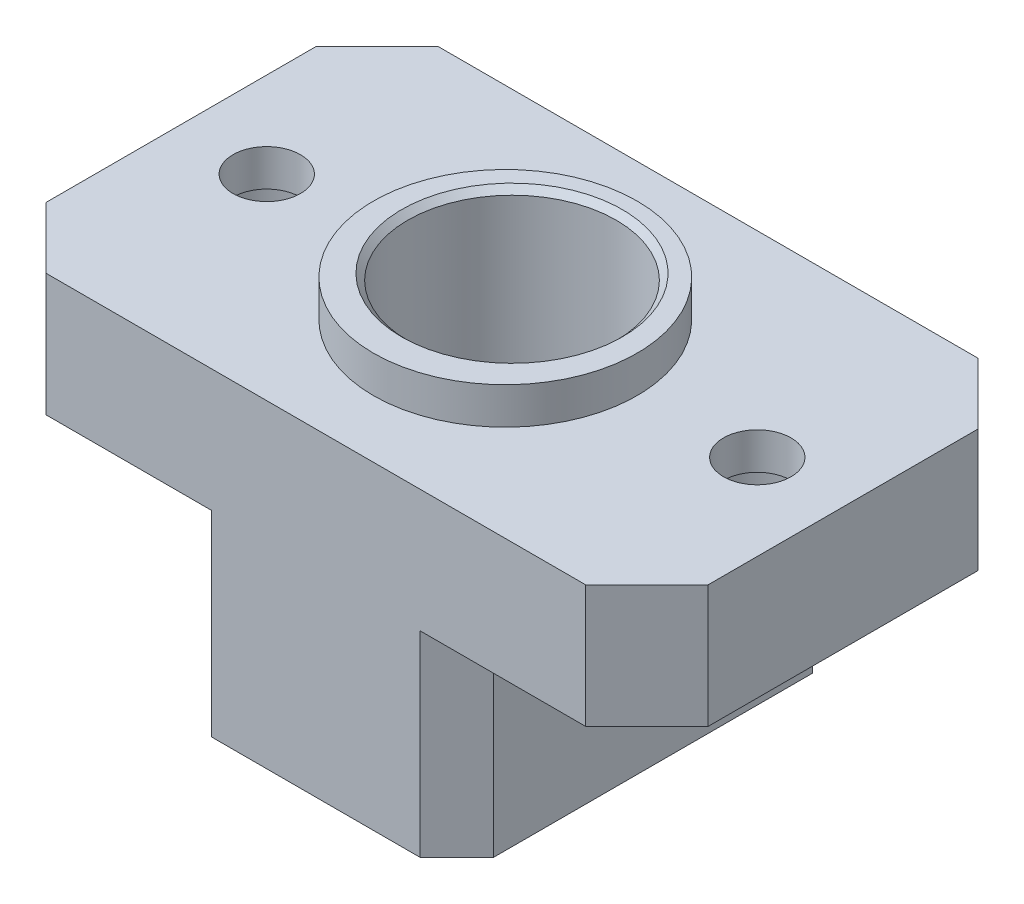
from build123d import *

# Parameters (mm, degrees)
BOSS_EXTRUDE1_DEPTH = 32
CHAMFER1_SIZE       = 5
SKETCH2_R           = 10.75
BOSS_EXTRUDE2_DEPTH = 3
HOLE2_D             = 5.5
HOLE2_DEPTH         = 100
HOLE2_CBORE_D       = 10
HOLE2_CBORE_DEPTH   = 7
CHAMFER3_SIZE       = 3
HOLE3_D             = 17
CHAMFER5_SIZE       = 0.5
CHAMFER6_SIZE       = 1


with BuildPart() as part:
    # Sketch1 → Boss-Extrude1 (new body)
    with BuildSketch(Plane.XY):
        Polygon((11.5, -16.008629624), (-11.5, -16.008629624), (-11.5, -0.008629624), (-27, -0.008629624), (-27, 9.991370376), (27, 9.991370376), (27, -0.008629624), (11.5, -0.008629624), align=None)
    extrude(amount=BOSS_EXTRUDE1_DEPTH)

    # Chamfer1
    chamfer1_edges = [part.edges().sort_by_distance(p)[0] for p in [
        (-27, 4.991370376, 0),
        (27, 4.991370376, 0),
        (-27, 4.991370376, 32),
        (27, 4.991370376, 32),
    ]]
    chamfer(chamfer1_edges, length=CHAMFER1_SIZE)

    # Sketch2 → Boss-Extrude2 (add)
    with BuildSketch(Plane(origin=(0, 9.991370376, 0), x_dir=(1, 0, 0), z_dir=(0, 1, 0))):
        with Locations(Location((0, -16.547126345, 0), (0, 0, 270))):
            Circle(SKETCH2_R)
    extrude(amount=BOSS_EXTRUDE2_DEPTH)

    # Hole2
    with Locations(Plane(origin=(0, -0.008629624, 0), x_dir=(-1, 0, 0), z_dir=(0, -1, 0))):
        with Locations((-20, -16), (20, -16)):
            CounterBoreHole(HOLE2_D / 2, HOLE2_CBORE_D / 2, HOLE2_CBORE_DEPTH, depth=HOLE2_DEPTH)

    # Chamfer3
    chamfer3_edges = [part.edges().sort_by_distance(p)[0] for p in [
        (-11.5, -8.008629624, 32),
        (11.5, -8.008629624, 32),
        (11.5, -8.008629624, 0),
        (-11.5, -8.008629624, 0),
    ]]
    chamfer(chamfer3_edges, length=CHAMFER3_SIZE)

    # Hole3 (through all)
    with Locations(Plane(origin=(0, -16.008629624, 0), x_dir=(-1, 0, 0), z_dir=(0, -1, 0))):
        with Locations((0, -16)):
            Hole(HOLE3_D / 2)

    # Chamfer5
    chamfer5_edges = [part.edges().sort_by_distance(p)[0] for p in [
        (-8.5, 12.991370376, 16),
    ]]
    chamfer(chamfer5_edges, length=CHAMFER5_SIZE)

    # Chamfer6
    chamfer6_edges = [part.edges().sort_by_distance(p)[0] for p in [
        (-8.5, -16.008629624, 16),
    ]]
    chamfer(chamfer6_edges, length=CHAMFER6_SIZE)


solid = part.part
